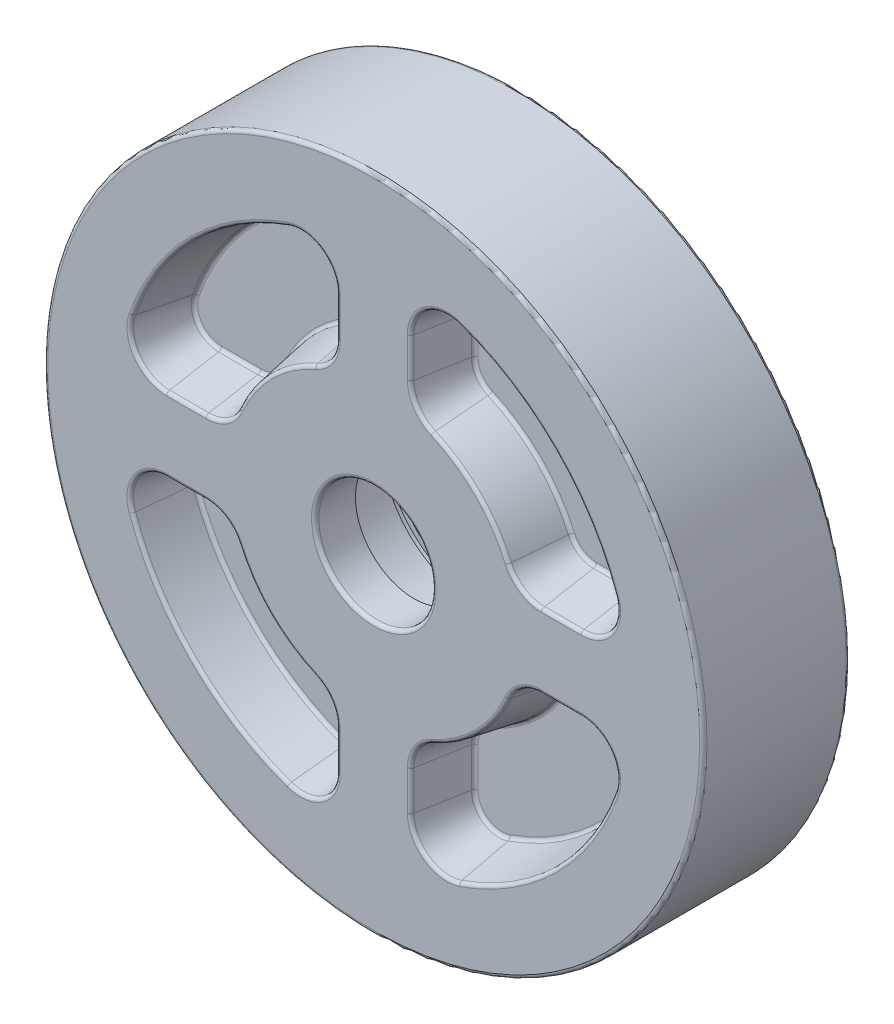
from build123d import *

# Parameters (mm, degrees)
SKETCH1_R                = 90
BOSS_EXTRUDE1_DEPTH      = 20
SKETCH2_R                = 16
CUT_EXTRUDE1_DEPTH       = 11
SKETCH3_R                = 22.5
CUT_EXTRUDE2_DEPTH       = 2
SKETCH4_R                = 26
CUT_EXTRUDE3_DEPTH       = 15
SKETCH5_R                = 27.5
CUT_EXTRUDE4_DEPTH       = 2
SKETCH6_R                = 26
CUT_EXTRUDE5_DEPTH       = 131.766968306
CUT_EXTRUDE6_DEPTH       = 15
CUT_EXTRUDE6_DRAFT       = -10
CIRPATTERN1_COPY_1_DEPTH = 15
CIRPATTERN1_COPY_1_DRAFT = -10
CIRPATTERN1_COPY_2_DEPTH = 15
CIRPATTERN1_COPY_2_DRAFT = -10
CIRPATTERN1_COPY_3_DEPTH = 15
CIRPATTERN1_COPY_3_DRAFT = -10
MIRROR1_COPY_1_DEPTH     = 15
MIRROR1_COPY_1_DRAFT     = -10
MIRROR1_COPY_2_DEPTH     = 15
MIRROR1_COPY_2_DRAFT     = -10
MIRROR1_COPY_3_DEPTH     = 15
MIRROR1_COPY_3_DRAFT     = -10
MIRROR1_COPY_4_DEPTH     = 15
MIRROR1_COPY_4_DRAFT     = -10
FILLET1_R                = 1
FILLET2_R                = 1
SKETCH8_R                = 1.5
CUT_EXTRUDE7_DEPTH       = 10


with BuildPart() as part:
    # Sketch1 → Boss-Extrude1 (new, symmetric)
    with BuildSketch(Plane.XY):
        Circle(SKETCH1_R)
    extrude(amount=BOSS_EXTRUDE1_DEPTH, both=True)

    # Sketch2 → Cut-Extrude1 (cut)
    with BuildSketch(Plane.XY.offset(20)):
        Circle(SKETCH2_R)
    extrude(amount=-CUT_EXTRUDE1_DEPTH, mode=Mode.SUBTRACT)

    # Sketch3 → Cut-Extrude2 (cut)
    with BuildSketch(Plane.XY.offset(9)):
        Circle(SKETCH3_R)
    extrude(amount=-CUT_EXTRUDE2_DEPTH, mode=Mode.SUBTRACT)

    # Sketch4 → Cut-Extrude3 (cut)
    with BuildSketch(Plane.XY.offset(7)):
        Circle(SKETCH4_R)
    extrude(amount=-CUT_EXTRUDE3_DEPTH, mode=Mode.SUBTRACT)

    # Sketch5 → Cut-Extrude4 (cut)
    with BuildSketch(Plane.XY.offset(-8)):
        Circle(SKETCH5_R)
    extrude(amount=-CUT_EXTRUDE4_DEPTH, mode=Mode.SUBTRACT)

    # Sketch6 → Cut-Extrude5 (cut, through all)
    with BuildSketch(Plane.XY.offset(-10)):
        Circle(SKETCH6_R)
    extrude(amount=-CUT_EXTRUDE5_DEPTH, mode=Mode.SUBTRACT)


with BuildPart() as cut_extrude6_tool:
    # Sketch7 → Cut-Extrude6 (with draft: the straight prism first)
    with BuildSketch(Plane(origin=(0, 0, -20), x_dir=(-1, 0, 0), z_dir=(0, 0, -1))):
        with BuildLine():
            ThreePointArc((-10, 56.568542495), (-14.226497308, 64.733508304), (-23.333333333, 65.996632911))
            ThreePointArc((-23.333333333, 65.996632911), (-49.497474683, 49.497474683), (-65.996632911, 23.333333333))
            ThreePointArc((-65.996632911, 23.333333333), (-64.733508304, 14.226497308), (-56.568542495, 10))
            Line((-56.568542495, 10), (-45.82575695, 10))
            ThreePointArc((-45.82575695, 10), (-40.348531375, 11.633399735), (-36.66060556, 16))
            ThreePointArc((-36.66060556, 16), (-28.284271247, 28.284271247), (-16, 36.66060556))
            ThreePointArc((-16, 36.66060556), (-11.633399735, 40.348531375), (-10, 45.82575695))
            Line((-10, 45.82575695), (-10, 56.568542495))
        make_face()
    extrude(amount=-CUT_EXTRUDE6_DEPTH)
    # Cut-Extrude6: the draft: its side faces are tilted about the plane it starts from
    cut_extrude6_sides = [cut_extrude6_tool.faces().sort_by_distance(p)[0] for p in [
        (11.633399735, 40.348531375, -12.5),
        (10, 51.197149722, -12.5),
        (14.226497308, 64.733508304, -12.5),
        (49.497474683, 49.497474683, -12.5),
        (64.733508304, 14.226497308, -12.5),
        (51.197149722, 10, -12.5),
        (40.348531375, 11.633399735, -12.5),
        (28.284271247, 28.284271247, -12.5),
    ]]
    draft(cut_extrude6_sides, Plane(origin=(0, 0, -20), x_dir=(-1, 0, 0), z_dir=(0, 0, -1)), CUT_EXTRUDE6_DRAFT)


with BuildPart() as part_1:
    add(part.part)

    # Cut-Extrude6: cut by cut_extrude6_tool
    add(cut_extrude6_tool.part, mode=Mode.SUBTRACT)


with BuildPart() as cirpattern1_copy_1_tool:
    # CirPattern1 copy 1 sketch → CirPattern1 copy 1 (with draft: the straight prism first)
    with BuildSketch(Plane(origin=(0, 0, -20), x_dir=(0, -1, 0), z_dir=(0, 0, -1))):
        with BuildLine():
            ThreePointArc((-10, 56.568542495), (-14.226497308, 64.733508304), (-23.333333333, 65.996632911))
            ThreePointArc((-23.333333333, 65.996632911), (-49.497474683, 49.497474683), (-65.996632911, 23.333333333))
            ThreePointArc((-65.996632911, 23.333333333), (-64.733508304, 14.226497308), (-56.568542495, 10))
            Line((-56.568542495, 10), (-45.82575695, 10))
            ThreePointArc((-45.82575695, 10), (-40.348531375, 11.633399735), (-36.66060556, 16))
            ThreePointArc((-36.66060556, 16), (-28.284271247, 28.284271247), (-16, 36.66060556))
            ThreePointArc((-16, 36.66060556), (-11.633399735, 40.348531375), (-10, 45.82575695))
            Line((-10, 45.82575695), (-10, 56.568542495))
        make_face()
    extrude(amount=-CIRPATTERN1_COPY_1_DEPTH)
    # CirPattern1 copy 1: the draft: its side faces are tilted about the plane it starts from
    cirpattern1_copy_1_sides = [cirpattern1_copy_1_tool.faces().sort_by_distance(p)[0] for p in [
        (-40.348531375, 11.633399735, -12.5),
        (-51.197149722, 10, -12.5),
        (-64.733508304, 14.226497308, -12.5),
        (-49.497474683, 49.497474683, -12.5),
        (-14.226497308, 64.733508304, -12.5),
        (-10, 51.197149722, -12.5),
        (-11.633399735, 40.348531375, -12.5),
        (-28.284271247, 28.284271247, -12.5),
    ]]
    draft(cirpattern1_copy_1_sides, Plane(origin=(0, 0, -20), x_dir=(0, -1, 0), z_dir=(0, 0, -1)), CIRPATTERN1_COPY_1_DRAFT)


with BuildPart() as part_2:
    add(part_1.part)

    # CirPattern1 copy 1: cut by cirpattern1_copy_1_tool
    add(cirpattern1_copy_1_tool.part, mode=Mode.SUBTRACT)


with BuildPart() as cirpattern1_copy_2_tool:
    # CirPattern1 copy 2 sketch → CirPattern1 copy 2 (with draft: the straight prism first)
    with BuildSketch(Plane(origin=(0, 0, -20), x_dir=(1, 0, 0), z_dir=(0, 0, -1))):
        with BuildLine():
            ThreePointArc((-10, 56.568542495), (-14.226497308, 64.733508304), (-23.333333333, 65.996632911))
            ThreePointArc((-23.333333333, 65.996632911), (-49.497474683, 49.497474683), (-65.996632911, 23.333333333))
            ThreePointArc((-65.996632911, 23.333333333), (-64.733508304, 14.226497308), (-56.568542495, 10))
            Line((-56.568542495, 10), (-45.82575695, 10))
            ThreePointArc((-45.82575695, 10), (-40.348531375, 11.633399735), (-36.66060556, 16))
            ThreePointArc((-36.66060556, 16), (-28.284271247, 28.284271247), (-16, 36.66060556))
            ThreePointArc((-16, 36.66060556), (-11.633399735, 40.348531375), (-10, 45.82575695))
            Line((-10, 45.82575695), (-10, 56.568542495))
        make_face()
    extrude(amount=-CIRPATTERN1_COPY_2_DEPTH)
    # CirPattern1 copy 2: the draft: its side faces are tilted about the plane it starts from
    cirpattern1_copy_2_sides = [cirpattern1_copy_2_tool.faces().sort_by_distance(p)[0] for p in [
        (-11.633399735, -40.348531375, -12.5),
        (-10, -51.197149722, -12.5),
        (-14.226497308, -64.733508304, -12.5),
        (-49.497474683, -49.497474683, -12.5),
        (-64.733508304, -14.226497308, -12.5),
        (-51.197149722, -10, -12.5),
        (-40.348531375, -11.633399735, -12.5),
        (-28.284271247, -28.284271247, -12.5),
    ]]
    draft(cirpattern1_copy_2_sides, Plane(origin=(0, 0, -20), x_dir=(1, 0, 0), z_dir=(0, 0, -1)), CIRPATTERN1_COPY_2_DRAFT)


with BuildPart() as part_3:
    add(part_2.part)

    # CirPattern1 copy 2: cut by cirpattern1_copy_2_tool
    add(cirpattern1_copy_2_tool.part, mode=Mode.SUBTRACT)


with BuildPart() as cirpattern1_copy_3_tool:
    # CirPattern1 copy 3 sketch → CirPattern1 copy 3 (with draft: the straight prism first)
    with BuildSketch(Plane.YX.offset(20)):
        with BuildLine():
            ThreePointArc((-10, 56.568542495), (-14.226497308, 64.733508304), (-23.333333333, 65.996632911))
            ThreePointArc((-23.333333333, 65.996632911), (-49.497474683, 49.497474683), (-65.996632911, 23.333333333))
            ThreePointArc((-65.996632911, 23.333333333), (-64.733508304, 14.226497308), (-56.568542495, 10))
            Line((-56.568542495, 10), (-45.82575695, 10))
            ThreePointArc((-45.82575695, 10), (-40.348531375, 11.633399735), (-36.66060556, 16))
            ThreePointArc((-36.66060556, 16), (-28.284271247, 28.284271247), (-16, 36.66060556))
            ThreePointArc((-16, 36.66060556), (-11.633399735, 40.348531375), (-10, 45.82575695))
            Line((-10, 45.82575695), (-10, 56.568542495))
        make_face()
    extrude(amount=-CIRPATTERN1_COPY_3_DEPTH)
    # CirPattern1 copy 3: the draft: its side faces are tilted about the plane it starts from
    cirpattern1_copy_3_sides = [cirpattern1_copy_3_tool.faces().sort_by_distance(p)[0] for p in [
        (40.348531375, -11.633399735, -12.5),
        (51.197149722, -10, -12.5),
        (64.733508304, -14.226497308, -12.5),
        (49.497474683, -49.497474683, -12.5),
        (14.226497308, -64.733508304, -12.5),
        (10, -51.197149722, -12.5),
        (11.633399735, -40.348531375, -12.5),
        (28.284271247, -28.284271247, -12.5),
    ]]
    draft(cirpattern1_copy_3_sides, Plane.YX.offset(20), CIRPATTERN1_COPY_3_DRAFT)


with BuildPart() as part_4:
    add(part_3.part)

    # CirPattern1 copy 3: cut by cirpattern1_copy_3_tool
    add(cirpattern1_copy_3_tool.part, mode=Mode.SUBTRACT)


with BuildPart() as mirror1_copy_1_tool:
    # Mirror1 copy 1 sketch → Mirror1 copy 1 (with draft: the straight prism first)
    with BuildSketch(Plane(origin=(0, 0, 20), x_dir=(-1, 0, 0), z_dir=(0, 0, 1))):
        with BuildLine():
            ThreePointArc((-10, -56.568542495), (-14.226497308, -64.733508304), (-23.333333333, -65.996632911))
            ThreePointArc((-23.333333333, -65.996632911), (-49.497474683, -49.497474683), (-65.996632911, -23.333333333))
            ThreePointArc((-65.996632911, -23.333333333), (-64.733508304, -14.226497308), (-56.568542495, -10))
            Line((-56.568542495, -10), (-45.82575695, -10))
            ThreePointArc((-45.82575695, -10), (-40.348531375, -11.633399735), (-36.66060556, -16))
            ThreePointArc((-36.66060556, -16), (-28.284271247, -28.284271247), (-16, -36.66060556))
            ThreePointArc((-16, -36.66060556), (-11.633399735, -40.348531375), (-10, -45.82575695))
            Line((-10, -45.82575695), (-10, -56.568542495))
        make_face()
    extrude(amount=-MIRROR1_COPY_1_DEPTH)
    # Mirror1 copy 1: the draft: its side faces are tilted about the plane it starts from
    mirror1_copy_1_sides = [mirror1_copy_1_tool.faces().sort_by_distance(p)[0] for p in [
        (11.633399735, 40.348531375, 12.5),
        (10, 51.197149722, 12.5),
        (14.226497308, 64.733508304, 12.5),
        (49.497474683, 49.497474683, 12.5),
        (64.733508304, 14.226497308, 12.5),
        (51.197149722, 10, 12.5),
        (40.348531375, 11.633399735, 12.5),
        (28.284271247, 28.284271247, 12.5),
    ]]
    draft(mirror1_copy_1_sides, Plane(origin=(0, 0, 20), x_dir=(-1, 0, 0), z_dir=(0, 0, 1)), MIRROR1_COPY_1_DRAFT)


with BuildPart() as part_5:
    add(part_4.part)

    # Mirror1 copy 1: cut by mirror1_copy_1_tool
    add(mirror1_copy_1_tool.part, mode=Mode.SUBTRACT)


with BuildPart() as mirror1_copy_2_tool:
    # Mirror1 copy 2 sketch → Mirror1 copy 2 (with draft: the straight prism first)
    with BuildSketch(Plane(origin=(0, 0, 20), x_dir=(0, -1, 0), z_dir=(0, 0, 1))):
        with BuildLine():
            ThreePointArc((-10, -56.568542495), (-14.226497308, -64.733508304), (-23.333333333, -65.996632911))
            ThreePointArc((-23.333333333, -65.996632911), (-49.497474683, -49.497474683), (-65.996632911, -23.333333333))
            ThreePointArc((-65.996632911, -23.333333333), (-64.733508304, -14.226497308), (-56.568542495, -10))
            Line((-56.568542495, -10), (-45.82575695, -10))
            ThreePointArc((-45.82575695, -10), (-40.348531375, -11.633399735), (-36.66060556, -16))
            ThreePointArc((-36.66060556, -16), (-28.284271247, -28.284271247), (-16, -36.66060556))
            ThreePointArc((-16, -36.66060556), (-11.633399735, -40.348531375), (-10, -45.82575695))
            Line((-10, -45.82575695), (-10, -56.568542495))
        make_face()
    extrude(amount=-MIRROR1_COPY_2_DEPTH)
    # Mirror1 copy 2: the draft: its side faces are tilted about the plane it starts from
    mirror1_copy_2_sides = [mirror1_copy_2_tool.faces().sort_by_distance(p)[0] for p in [
        (-40.348531375, 11.633399735, 12.5),
        (-51.197149722, 10, 12.5),
        (-64.733508304, 14.226497308, 12.5),
        (-49.497474683, 49.497474683, 12.5),
        (-14.226497308, 64.733508304, 12.5),
        (-10, 51.197149722, 12.5),
        (-11.633399735, 40.348531375, 12.5),
        (-28.284271247, 28.284271247, 12.5),
    ]]
    draft(mirror1_copy_2_sides, Plane(origin=(0, 0, 20), x_dir=(0, -1, 0), z_dir=(0, 0, 1)), MIRROR1_COPY_2_DRAFT)


with BuildPart() as part_6:
    add(part_5.part)

    # Mirror1 copy 2: cut by mirror1_copy_2_tool
    add(mirror1_copy_2_tool.part, mode=Mode.SUBTRACT)


with BuildPart() as mirror1_copy_3_tool:
    # Mirror1 copy 3 sketch → Mirror1 copy 3 (with draft: the straight prism first)
    with BuildSketch(Plane.XY.offset(20)):
        with BuildLine():
            ThreePointArc((-10, -56.568542495), (-14.226497308, -64.733508304), (-23.333333333, -65.996632911))
            ThreePointArc((-23.333333333, -65.996632911), (-49.497474683, -49.497474683), (-65.996632911, -23.333333333))
            ThreePointArc((-65.996632911, -23.333333333), (-64.733508304, -14.226497308), (-56.568542495, -10))
            Line((-56.568542495, -10), (-45.82575695, -10))
            ThreePointArc((-45.82575695, -10), (-40.348531375, -11.633399735), (-36.66060556, -16))
            ThreePointArc((-36.66060556, -16), (-28.284271247, -28.284271247), (-16, -36.66060556))
            ThreePointArc((-16, -36.66060556), (-11.633399735, -40.348531375), (-10, -45.82575695))
            Line((-10, -45.82575695), (-10, -56.568542495))
        make_face()
    extrude(amount=-MIRROR1_COPY_3_DEPTH)
    # Mirror1 copy 3: the draft: its side faces are tilted about the plane it starts from
    mirror1_copy_3_sides = [mirror1_copy_3_tool.faces().sort_by_distance(p)[0] for p in [
        (-11.633399735, -40.348531375, 12.5),
        (-10, -51.197149722, 12.5),
        (-14.226497308, -64.733508304, 12.5),
        (-49.497474683, -49.497474683, 12.5),
        (-64.733508304, -14.226497308, 12.5),
        (-51.197149722, -10, 12.5),
        (-40.348531375, -11.633399735, 12.5),
        (-28.284271247, -28.284271247, 12.5),
    ]]
    draft(mirror1_copy_3_sides, Plane.XY.offset(20), MIRROR1_COPY_3_DRAFT)


with BuildPart() as part_7:
    add(part_6.part)

    # Mirror1 copy 3: cut by mirror1_copy_3_tool
    add(mirror1_copy_3_tool.part, mode=Mode.SUBTRACT)


with BuildPart() as mirror1_copy_4_tool:
    # Mirror1 copy 4 sketch → Mirror1 copy 4 (with draft: the straight prism first)
    with BuildSketch(Plane(origin=(0, 0, 20), x_dir=(0, 1, 0), z_dir=(0, 0, 1))):
        with BuildLine():
            ThreePointArc((-10, -56.568542495), (-14.226497308, -64.733508304), (-23.333333333, -65.996632911))
            ThreePointArc((-23.333333333, -65.996632911), (-49.497474683, -49.497474683), (-65.996632911, -23.333333333))
            ThreePointArc((-65.996632911, -23.333333333), (-64.733508304, -14.226497308), (-56.568542495, -10))
            Line((-56.568542495, -10), (-45.82575695, -10))
            ThreePointArc((-45.82575695, -10), (-40.348531375, -11.633399735), (-36.66060556, -16))
            ThreePointArc((-36.66060556, -16), (-28.284271247, -28.284271247), (-16, -36.66060556))
            ThreePointArc((-16, -36.66060556), (-11.633399735, -40.348531375), (-10, -45.82575695))
            Line((-10, -45.82575695), (-10, -56.568542495))
        make_face()
    extrude(amount=-MIRROR1_COPY_4_DEPTH)
    # Mirror1 copy 4: the draft: its side faces are tilted about the plane it starts from
    mirror1_copy_4_sides = [mirror1_copy_4_tool.faces().sort_by_distance(p)[0] for p in [
        (40.348531375, -11.633399735, 12.5),
        (51.197149722, -10, 12.5),
        (64.733508304, -14.226497308, 12.5),
        (49.497474683, -49.497474683, 12.5),
        (14.226497308, -64.733508304, 12.5),
        (10, -51.197149722, 12.5),
        (11.633399735, -40.348531375, 12.5),
        (28.284271247, -28.284271247, 12.5),
    ]]
    draft(mirror1_copy_4_sides, Plane(origin=(0, 0, 20), x_dir=(0, 1, 0), z_dir=(0, 0, 1)), MIRROR1_COPY_4_DRAFT)


with BuildPart() as part_8:
    add(part_7.part)

    # Mirror1 copy 4: cut by mirror1_copy_4_tool
    add(mirror1_copy_4_tool.part, mode=Mode.SUBTRACT)

    # Fillet1
    fillet1_edges = [part_8.edges().sort_by_distance(p)[0] for p in [
        (64.733508304, 14.226497308, 20),
        (51.197149722, 10, 20),
        (40.348531375, 11.633399735, 20),
        (28.284271247, 28.284271247, 20),
        (11.633399735, 40.348531375, 20),
        (10, 51.197149722, 20),
        (14.226497308, 64.733508304, 20),
        (49.497474683, 49.497474683, 20),
        (62.573952651, 15.753533755, 5),
        (51.197149722, 12.644904711, 5),
        (41.797205347, 13.84628578, 5),
        (30.154501304, 30.154501304, 5),
        (13.84628578, 41.797205347, 5),
        (12.644904711, 51.197149722, 5),
        (15.753533755, 62.573952651, 5),
        (47.627244627, 47.627244627, 5),
        (14.226497308, -64.733508304, 20),
        (10, -51.197149722, 20),
        (11.633399735, -40.348531375, 20),
        (28.284271247, -28.284271247, 20),
        (40.348531375, -11.633399735, 20),
        (51.197149722, -10, 20),
        (64.733508304, -14.226497308, 20),
        (49.497474683, -49.497474683, 20),
        (15.753533755, -62.573952651, 5),
        (12.644904711, -51.197149722, 5),
        (13.84628578, -41.797205347, 5),
        (30.154501304, -30.154501304, 5),
        (41.797205347, -13.84628578, 5),
        (51.197149722, -12.644904711, 5),
        (62.573952651, -15.753533755, 5),
        (47.627244627, -47.627244627, 5),
        (-64.733508304, -14.226497308, 20),
        (-51.197149722, -10, 20),
        (-40.348531375, -11.633399735, 20),
        (-28.284271247, -28.284271247, 20),
        (-11.633399735, -40.348531375, 20),
        (-10, -51.197149722, 20),
        (-14.226497308, -64.733508304, 20),
        (-49.497474683, -49.497474683, 20),
        (-62.573952651, -15.753533755, 5),
        (-51.197149722, -12.644904711, 5),
        (-41.797205347, -13.84628578, 5),
        (-30.154501304, -30.154501304, 5),
        (-13.84628578, -41.797205347, 5),
        (-12.644904711, -51.197149722, 5),
        (-15.753533755, -62.573952651, 5),
        (-47.627244627, -47.627244627, 5),
        (-14.226497308, 64.733508304, 20),
        (-10, 51.197149722, 20),
        (-11.633399735, 40.348531375, 20),
        (-28.284271247, 28.284271247, 20),
        (-40.348531375, 11.633399735, 20),
        (-51.197149722, 10, 20),
        (-64.733508304, 14.226497308, 20),
        (-49.497474683, 49.497474683, 20),
        (-15.753533755, 62.573952651, 5),
        (-12.644904711, 51.197149722, 5),
        (-13.84628578, 41.797205347, 5),
        (-30.154501304, 30.154501304, 5),
        (-41.797205347, 13.84628578, 5),
        (-51.197149722, 12.644904711, 5),
        (-62.573952651, 15.753533755, 5),
        (-47.627244627, 47.627244627, 5),
        (-90, 0, 20),
        (-16, 0, 20),
    ]]
    fillet(fillet1_edges, radius=FILLET1_R)

    # Fillet2
    fillet2_edges = [part_8.edges().sort_by_distance(p)[0] for p in [
        (-90, 0, -20),
        (-26, 0, -20),
        (62.573952651, 15.753533755, -5),
        (47.627244627, 47.627244627, -5),
        (15.753533755, 62.573952651, -5),
        (12.644904711, 51.197149722, -5),
        (13.84628578, 41.797205347, -5),
        (30.154501304, 30.154501304, -5),
        (41.797205347, 13.84628578, -5),
        (51.197149722, 12.644904711, -5),
        (64.733508304, 14.226497308, -20),
        (51.197149722, 10, -20),
        (40.348531375, 11.633399735, -20),
        (28.284271247, 28.284271247, -20),
        (11.633399735, 40.348531375, -20),
        (10, 51.197149722, -20),
        (14.226497308, 64.733508304, -20),
        (49.497474683, 49.497474683, -20),
        (15.753533755, -62.573952651, -5),
        (47.627244627, -47.627244627, -5),
        (62.573952651, -15.753533755, -5),
        (51.197149722, -12.644904711, -5),
        (41.797205347, -13.84628578, -5),
        (30.154501304, -30.154501304, -5),
        (13.84628578, -41.797205347, -5),
        (12.644904711, -51.197149722, -5),
        (14.226497308, -64.733508304, -20),
        (10, -51.197149722, -20),
        (11.633399735, -40.348531375, -20),
        (28.284271247, -28.284271247, -20),
        (40.348531375, -11.633399735, -20),
        (51.197149722, -10, -20),
        (64.733508304, -14.226497308, -20),
        (49.497474683, -49.497474683, -20),
        (-62.573952651, -15.753533755, -5),
        (-47.627244627, -47.627244627, -5),
        (-15.753533755, -62.573952651, -5),
        (-12.644904711, -51.197149722, -5),
        (-13.84628578, -41.797205347, -5),
        (-30.154501304, -30.154501304, -5),
        (-41.797205347, -13.84628578, -5),
        (-51.197149722, -12.644904711, -5),
        (-64.733508304, -14.226497308, -20),
        (-51.197149722, -10, -20),
        (-40.348531375, -11.633399735, -20),
        (-28.284271247, -28.284271247, -20),
        (-11.633399735, -40.348531375, -20),
        (-10, -51.197149722, -20),
        (-14.226497308, -64.733508304, -20),
        (-49.497474683, -49.497474683, -20),
        (-15.753533755, 62.573952651, -5),
        (-47.627244627, 47.627244627, -5),
        (-62.573952651, 15.753533755, -5),
        (-51.197149722, 12.644904711, -5),
        (-41.797205347, 13.84628578, -5),
        (-30.154501304, 30.154501304, -5),
        (-13.84628578, 41.797205347, -5),
        (-12.644904711, 51.197149722, -5),
        (-14.226497308, 64.733508304, -20),
        (-10, 51.197149722, -20),
        (-11.633399735, 40.348531375, -20),
        (-28.284271247, 28.284271247, -20),
        (-40.348531375, 11.633399735, -20),
        (-51.197149722, 10, -20),
        (-64.733508304, 14.226497308, -20),
        (-49.497474683, 49.497474683, -20),
    ]]
    fillet(fillet2_edges, radius=FILLET2_R)

    # Sketch8 → Cut-Extrude7 (cut)
    with BuildSketch(Plane(origin=(0, 0, -20), x_dir=(-1, 0, 0), z_dir=(0, 0, -1))):
        with Locations((0, 32.5)):
            Circle(SKETCH8_R)
        with Locations((28.145825623, -16.25)):
            Circle(SKETCH8_R)
        with Locations((-28.145825623, -16.25)):
            Circle(SKETCH8_R)
    extrude(amount=-CUT_EXTRUDE7_DEPTH, mode=Mode.SUBTRACT)


solid = part_8.part
